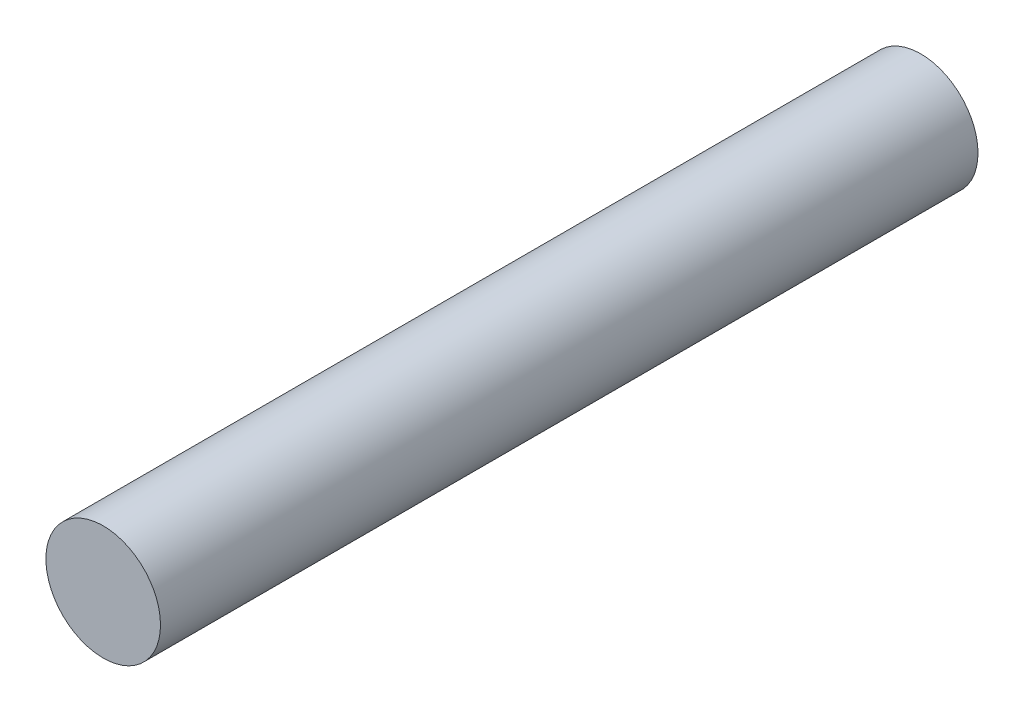
SolidWorks part; units mm, degrees
ref_plane "Front Plane" through (0, 0, 0) normal (0, 0, 1) x (1, 0, 0)
ref_plane "Top Plane" through (0, 0, 0) normal (0, 1, 0) x (1, 0, 0)
ref_plane "Right Plane" through (0, 0, 0) normal (1, 0, 0) x (0, 0, -1)
sketch "Sketch1" plane through (0, 0, 0) normal (0, 0, 1) x (1, 0, 0)
  circle A0 centre (0, 0) radius 7.5
  dimension "D1" = 15
extrude "Boss-Extrude1" add sketch "Sketch1" along normal blind 94 and the other way blind 13 contours A0
